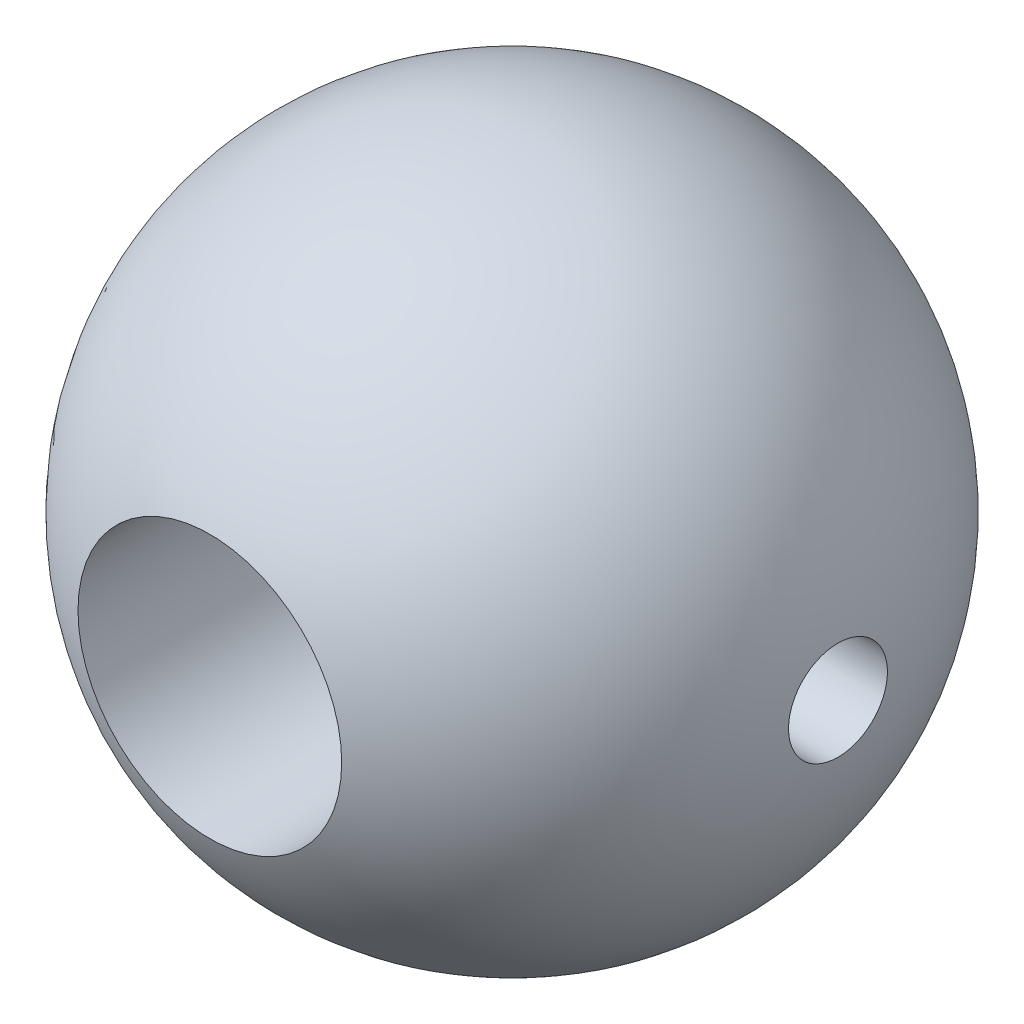
SolidWorks part; units mm, degrees
ref_plane "Front Plane" through (0, 0, 0) normal (0, 0, 1) x (1, 0, 0)
ref_plane "Top Plane" through (0, 0, 0) normal (0, 1, 0) x (1, 0, 0)
ref_plane "Right Plane" through (0, 0, 0) normal (1, 0, 0) x (0, 0, -1)
sketch "Sketch1" plane through (0, 0, 0) normal (0, 0, 1) x (1, 0, 0)
  line L0 (0, 10) -> (0, -10)
  arc A0 (0, 10) -> (0, -10) centre (0, 0) cw
  dimension "D1" = 10
revolve "Revolve1" add sketch "Sketch1" angle 360 about L0
sketch "Sketch2" plane through (0, 0, 0) normal (0, 0, 1) x (1, 0, 0)
  circle A0 centre (0, 0) radius 4
  dimension "D1" = 8
extrude "Cut-Extrude1" cut sketch "Sketch2" against normal mid plane 20
sketch "Sketch3" plane through (0, 0, 0) normal (1, 0, 0) x (0, 0, -1)
  circle A0 centre (0, 0) radius 1.5
  dimension "D1" = 3
extrude "Cut-Extrude2" cut sketch "Sketch3" against normal mid plane 30
